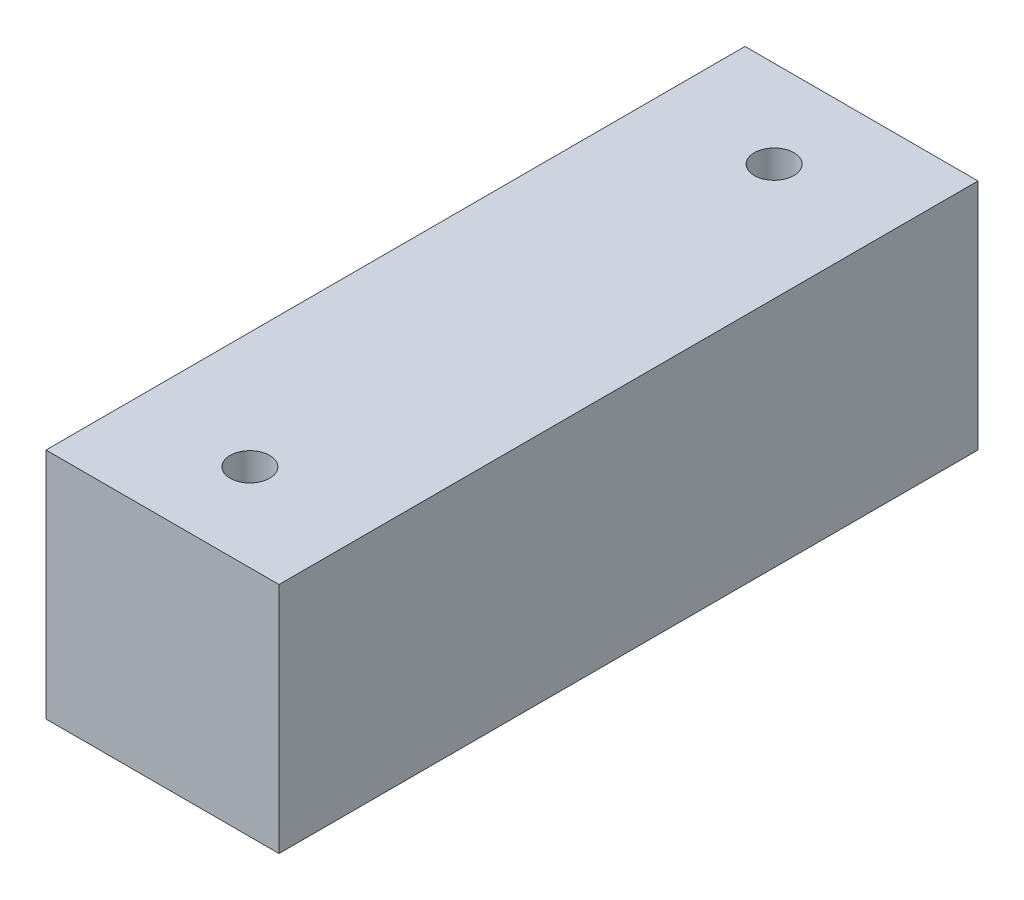
from build123d import *

# Parameters (mm, degrees)
SKETCH1_W           = 60
SKETCH1_H           = 60
BOSS_EXTRUDE1_DEPTH = 180
M12_TAPPED_HOLE1_D  = 10.2


with BuildPart() as part:
    # Sketch1 → Boss-Extrude1 (new body)
    with BuildSketch(Plane.XY):
        Rectangle(SKETCH1_W, SKETCH1_H)
    extrude(amount=BOSS_EXTRUDE1_DEPTH)

    # M12 Tapped Hole1 (through all)
    with Locations(Plane(origin=(0, 30, 0), x_dir=(1, 0, 0), z_dir=(0, 1, 0))):
        with Locations((0, -22.5), (0, -157.5)):
            Hole(M12_TAPPED_HOLE1_D / 2)


solid = part.part
